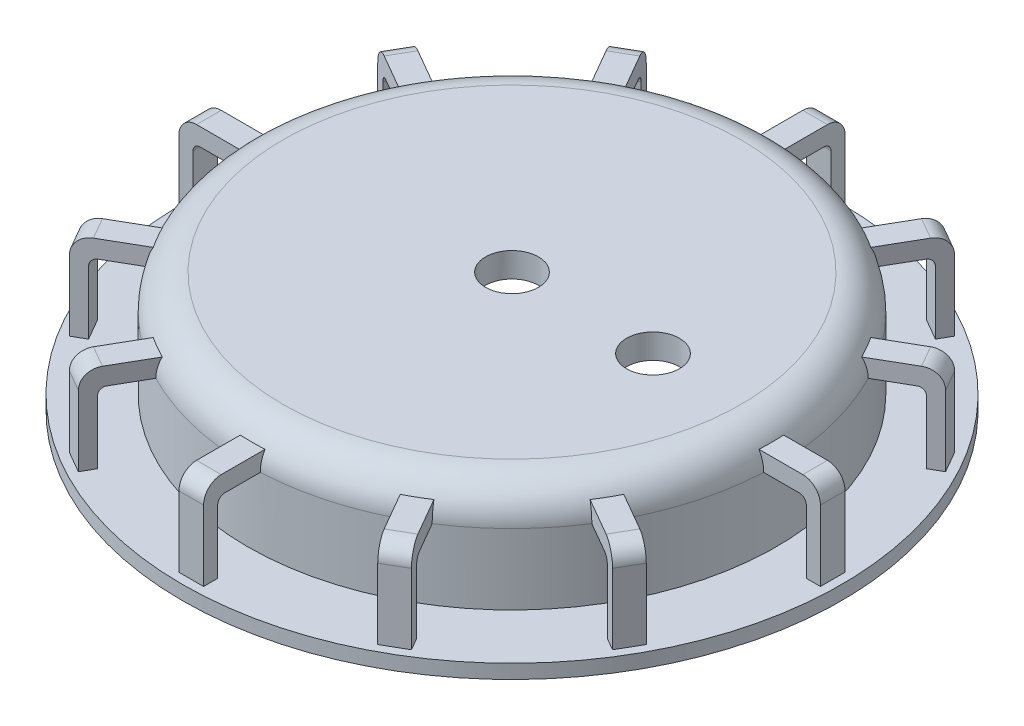
SolidWorks part; units mm, degrees
ref_plane "Front Plane" through (0, 0, 0) normal (0, 0, 1) x (1, 0, 0)
ref_plane "Top Plane" through (0, 0, 0) normal (0, 1, 0) x (1, 0, 0)
ref_plane "Right Plane" through (0, 0, 0) normal (1, 0, 0) x (0, 0, -1)
sketch "Sketch1" plane through (0, 0, 0) normal (0, 1, 0) x (1, 0, 0)
  circle A0 centre (0, 0) radius 75
  dimension "D1" = 150
extrude "Boss-Extrude1" add sketch "Sketch1" along normal blind 34
sketch "Sketch3" plane through (0, 0, 0) normal (0, 1, 0) x (1, 0, 0)
  circle A0 centre (0, 0) radius 93.5
  dimension "D1" = 187
extrude "Boss-Extrude2" add sketch "Sketch3" along normal blind 4
fillet "Fillet1" radius 10 1 edges at (0, 34, 75)
sketch "Sketch4" plane through (0, 0, 0) normal (0, -1, 0) x (1, 0, 0)
  circle A0 centre (0, 0) radius 50
  dimension "D1" = 100
extrude "Cut-Extrude1" cut sketch "Sketch4" against normal blind 27
sketch "Sketch6" plane through (0, 4, 0) normal (0, 1, 0) x (1, 0, 0)
  line L1 (87, 3.5) -> (91, 3.5)
  line L2 (87, 3.5) -> (87, -3.5)
  line L3 (87, -3.5) -> (91, -3.5)
  line L4 (91, 3.5) -> (91, -3.5)
  line L5 (87, 3.5) -> (91, -3.5) construction
  line L6 (87, -3.5) -> (91, 3.5) construction
  point P0 (89, 0)
  dimension "D1" = 89
  dimension "D2" = 4
  dimension "D3" = 7
extrude "Boss-Extrude3" add sketch "Sketch6" along normal blind 25
sketch "Sketch7" plane through (87, 0, 0) normal (-1, 0, 0) x (0, 0, 1)
  line L0 (3.5, 29) -> (3.5, 4) construction
  line L1 (-3.5, 29) -> (3.5, 29)
  line L2 (-3.5, 29) -> (-3.5, 24)
  line L3 (-3.5, 24) -> (3.5, 24)
  line L4 (3.5, 29) -> (3.5, 24)
  dimension "D1" = 5
extrude "Boss-Extrude4" add sketch "Sketch7" along normal up to surface (13.4229 mm away)
fillet "Fillet2" radius 5 1 edges at (91, 29, 0)
fillet "Fillet3" radius 2 1 edges at (87, 24, 0)
pattern_circular "CirPattern2" count 12 over 360 about axis through (0, 0, 0) along (0, 1, 0) of "Boss-Extrude4", "Boss-Extrude3", "Fillet2", "Fillet3"
sketch "Sketch8" plane through (0, 34, 0) normal (0, 1, 0) x (1, 0, 0)
  line L0 (0, 0) -> (0, 40.708) construction
  circle A0 centre (0, 0) radius 7.5
  circle A3 centre (40, 0) radius 7.5
  dimension "D1" = 15
  dimension "D2" = 40
  dimension "D3" = 15
extrude "Cut-Extrude2" cut sketch "Sketch8" against normal through all
